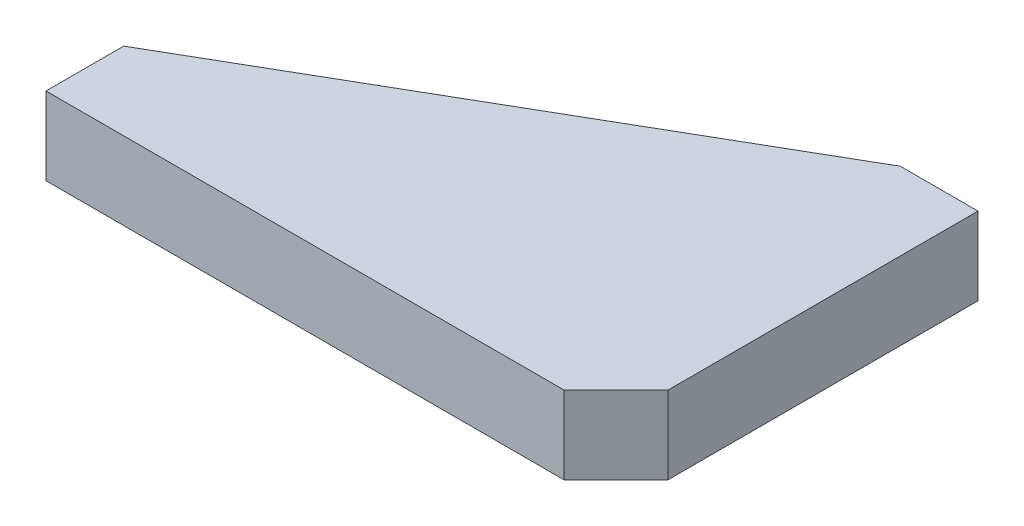
from build123d import *

# Parameters (mm, degrees)
EXTRUDE_1_DEPTH = 30


with BuildPart() as part:
    # 草图1 → 凸台-拉伸1 (new body)
    with BuildSketch(Plane(origin=(0, 0, 0), x_dir=(1, 0, 0), z_dir=(0, 1, 0))):
        Polygon((0, 0), (-30, 0), (-220, -109.696551146), (-220, -139.696551146), (-20, -139.696551146), (0, -119.696551146), align=None)
    extrude(amount=EXTRUDE_1_DEPTH)


solid = part.part
